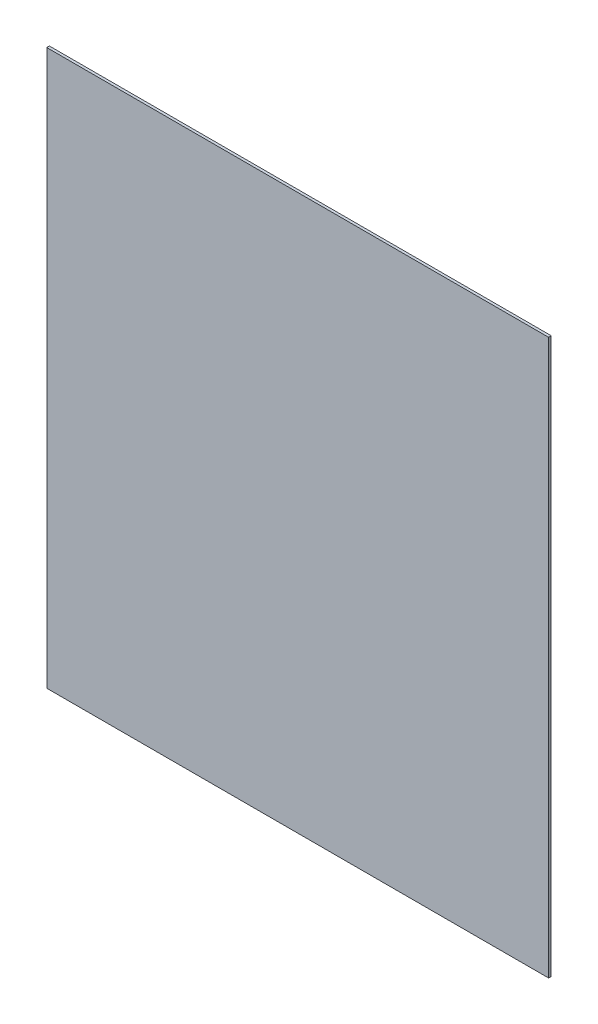
from build123d import *

# Parameters (mm, degrees)
SKETCH_1_W      = 1135
SKETCH_1_H      = 1255
EXTRUDE_1_DEPTH = 6


with BuildPart() as part:
    # 草图1 → 凸台-拉伸1 (new body)
    with BuildSketch(Plane.XY):
        Rectangle(SKETCH_1_W, SKETCH_1_H)
    extrude(amount=EXTRUDE_1_DEPTH)


solid = part.part
